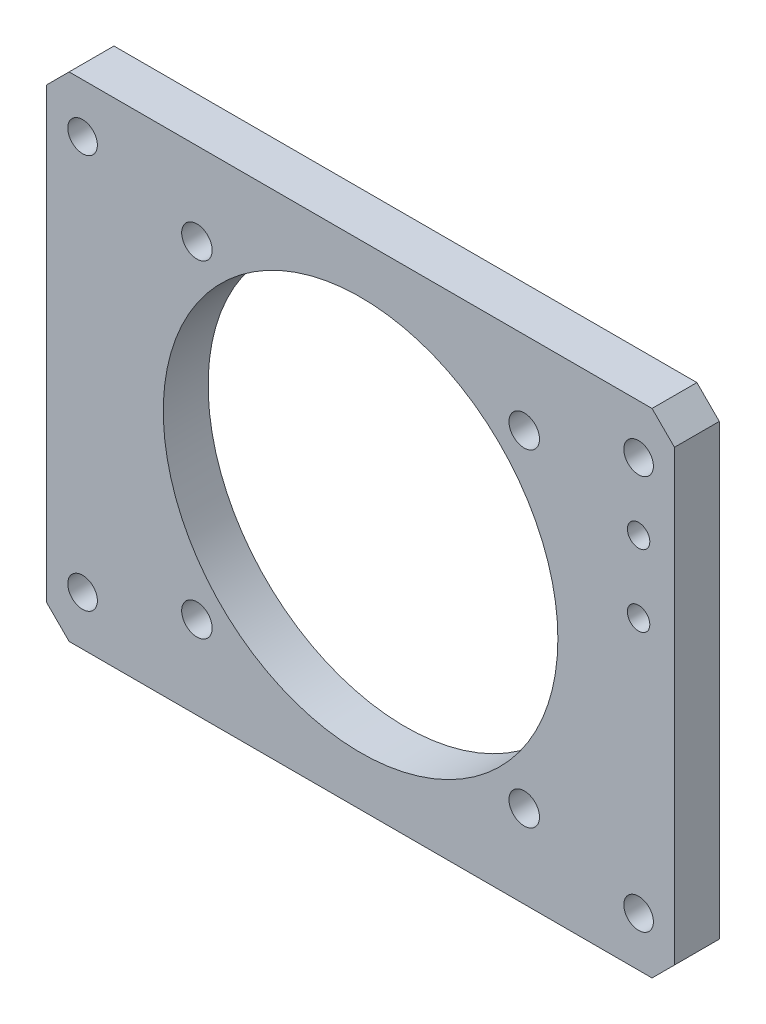
from build123d import *

# Parameters (mm, degrees)
SKETCH1_W           = 140
SKETCH1_H           = 110
SKETCH1_R           = 3.3
SKETCH1_R_2         = 44
BOSS_EXTRUDE1_DEPTH = 10
M8_TAPPED_HOLE1_D   = 6.8
CHAMFER1_SIZE       = 5
M6_TAPPED_HOLE1_D   = 5


with BuildPart() as part:
    # Sketch1 → Boss-Extrude1 (new body)
    with BuildSketch(Plane.XY):
        with Locations((5.534557186, 16.511254019)):
            Rectangle(SKETCH1_W, SKETCH1_H)
        with Locations((67.534557186, 60.511254019)):
            Circle(SKETCH1_R, mode=Mode.SUBTRACT)
        with Locations((67.534557186, -27.488745981)):
            Circle(SKETCH1_R, mode=Mode.SUBTRACT)
        with Locations((-56.465442814, -27.488745981)):
            Circle(SKETCH1_R, mode=Mode.SUBTRACT)
        with Locations((-56.465442814, 60.511254019)):
            Circle(SKETCH1_R, mode=Mode.SUBTRACT)
        with Locations((5.534557186, 16.511254019)):
            Circle(SKETCH1_R_2, mode=Mode.SUBTRACT)
    extrude(amount=BOSS_EXTRUDE1_DEPTH)

    # M8 Tapped Hole1 (through all)
    with Locations(Plane.XY.offset(10)):
        with Locations((-30.965442814, 53.011254019), (42.034557186, 53.011254019), (42.034557186, -19.988745981), (-30.965442814, -19.988745981)):
            Hole(M8_TAPPED_HOLE1_D / 2)

    # Chamfer1
    chamfer1_edges = [part.edges().sort_by_distance(p)[0] for p in [
        (75.534557186, -38.488745981, 5),
        (-64.465442814, -38.488745981, 5),
        (-64.465442814, 71.511254019, 5),
        (75.534557186, 71.511254019, 5),
    ]]
    chamfer(chamfer1_edges, length=CHAMFER1_SIZE)

    # M6 Tapped Hole1 (through all)
    with Locations(Plane.XY.offset(10)):
        with Locations((67.534557186, 45.511254019), (67.534557186, 29.511254019)):
            Hole(M6_TAPPED_HOLE1_D / 2)


solid = part.part
